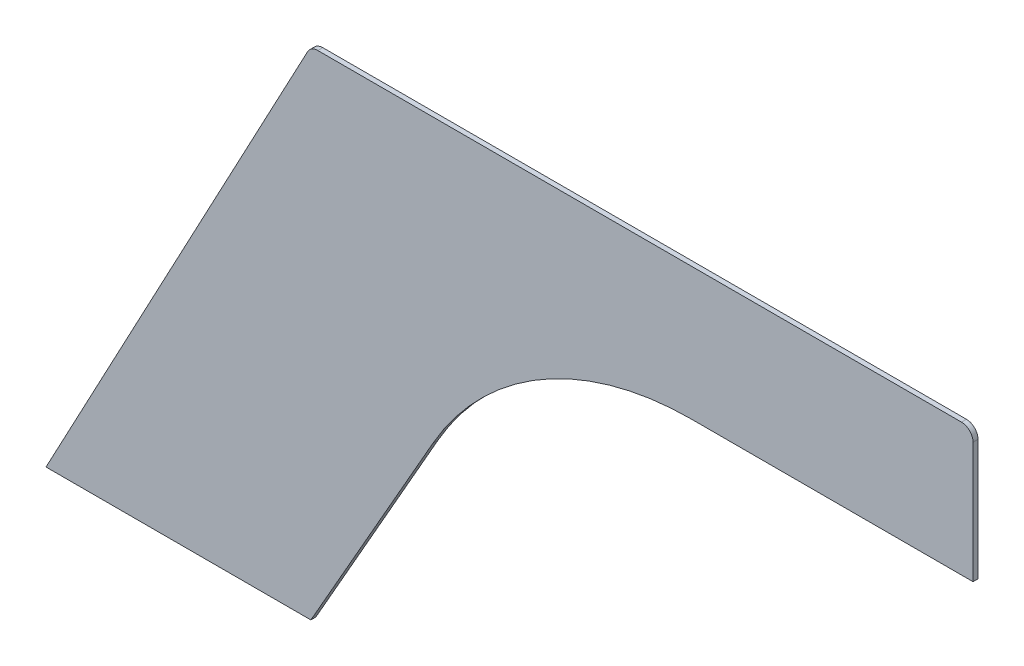
SolidWorks part; units mm, degrees
material "1023 Carbon Steel Plate (SS)"
ref_plane "Front Plane" through (0, 0, 0) normal (0, 0, 1) x (1, 0, 0)
ref_plane "Top Plane" through (0, 0, 0) normal (0, 1, 0) x (1, 0, 0)
ref_plane "Right Plane" through (0, 0, 0) normal (1, 0, 0) x (0, 0, -1)
sketch "Sketch1" plane through (0, 0, 0) normal (0, 0, 1) x (1, 0, 0)
  line L0 (0, 0) -> (79.0118, 148.1471)
  line L1 (82.1, 150) -> (276.5, 150)
  line L2 (280, 146.5) -> (280, 110)
  line L7 (80, 0) -> (0, 0)
  line L9 (195, 110) -> (280, 110)
  line L10 (80, 0) -> (116.8132, 64.5739)
  arc A0 (276.5, 150) -> (280, 146.5) centre (276.5, 146.5) cw
  arc A1 (79.0118, 148.1471) -> (82.1, 150) centre (82.1, 146.5) cw
  arc A4 (195, 110) -> (116.8132, 64.5739) centre (195, 20) ccw
  point P12 (280, 150)
  point P15 (80, 150)
  dimension "D9" = 3.5
  dimension "D5" = 90
  dimension "D1" = 80
  dimension "D2" = 200
  dimension "D3" = 200
  dimension "D4" = 85
  dimension "D6" = 150
  dimension "D8" = 40
extrude "Boss-Extrude1" add sketch "Sketch1" along normal blind 1.5 contours L7 L0 A1 L1 A0 L2 L9 A4 L10
